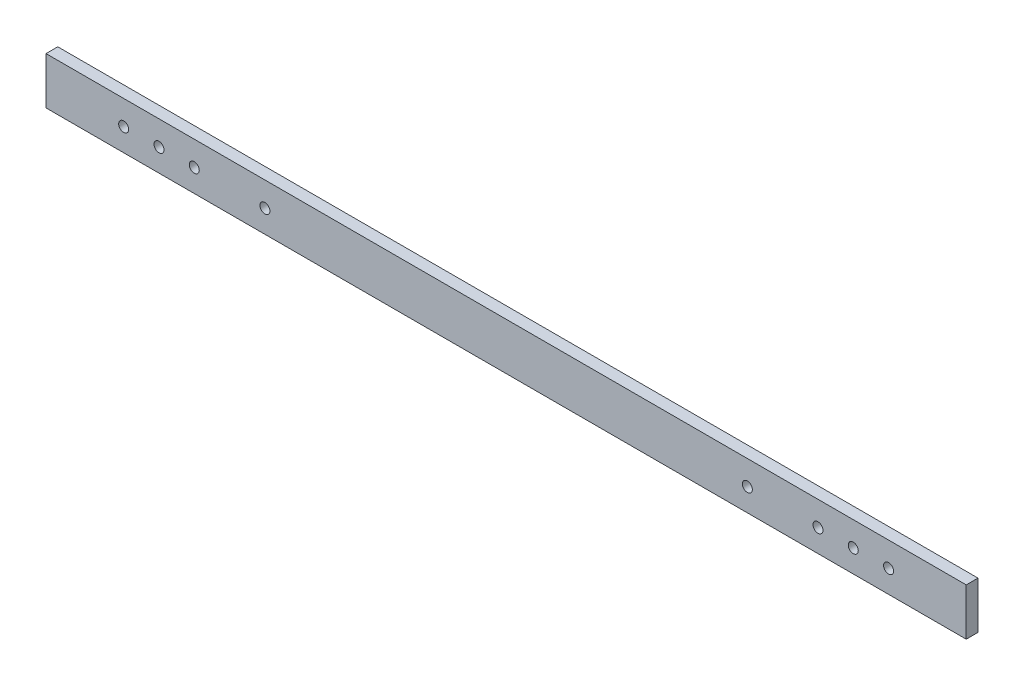
SolidWorks part; units mm, degrees
material "1023 carbon steel plate (SS)"
ref_plane "Front Plane" through (0, 0, 0) normal (0, 0, 1) x (1, 0, 0)
ref_plane "Top Plane" through (0, 0, 0) normal (0, 1, 0) x (1, 0, 0)
ref_plane "Right Plane" through (0, 0, 0) normal (1, 0, 0) x (0, 0, -1)
sketch "Sketch1" plane through (0, 0, 0) normal (0, 0, 1) x (1, 0, 0)
  line L1 (391, 20) -> (-391, 20)
  line L2 (391, 20) -> (391, -20)
  line L3 (391, -20) -> (-391, -20)
  line L4 (-391, 20) -> (-391, -20)
  line L5 (391, 20) -> (-391, -20) construction
  line L6 (391, -20) -> (-391, 20) construction
  point P0 (0, 0)
  dimension "D1" = 782
  dimension "D2" = 40
extrude "Boss-Extrude1" add sketch "Sketch1" along normal blind 10
sketch "Sketch2" plane through (0, 0, 10) normal (0, 0, 1) x (1, 0, 0)
  line L0 (-391, 20) -> (-391, -20) construction
  line L1 (0, 0) -> (0, 76.6808) construction
  line L2 (391, 20) -> (-391, 20) construction
  circle A0 centre (-325, -0.78) radius 4
  circle A1 centre (-295, -0.78) radius 4
  circle A2 centre (-265, -0.78) radius 4
  circle A3 centre (-205, -0.78) radius 4
  circle A12 centre (205, -0.78) radius 4
  circle A13 centre (265, -0.78) radius 4
  circle A14 centre (295, -0.78) radius 4
  circle A15 centre (325, -0.78) radius 4
  dimension "D1" = 8
  dimension "D6" = 20.78
  dimension "D2" = 30
  dimension "D3" = 66
  dimension "D4" = 30
  dimension "D5" = 60
hole_wizard "M10 Tapped Hole3" positions "Sketch7" profile "Sketch8" tap size "M10" standard "ISO"
sketch "Sketch7" plane through (0, 0, 10) normal (0, 0, 1) x (1, 0, 0)
  point P0 (-325, -0.78)
  point P3 (-295, -0.78)
  point P6 (-265, -0.78)
  point P9 (-205, -0.78)
  point P12 (205, -0.78)
  point P15 (265, -0.78)
  point P18 (295, -0.78)
  point P21 (325, -0.78)
sketch "Sketch8" plane through (-325, -0.78, 10) normal (1, 0, 0) x (0, -1, 0)
  line L0 (0, 0) -> (0, 27.0537)
  line L1 (0, 27.0537) -> (4.25, 24.5)
  line L2 (4.25, 24.5) -> (4.25, 0)
  line L5 (4.25, 0) -> (0, 0)
  line L10 (0, 27.0537) -> (-4.25, 24.5) construction
  line L11 (0, -6.35) -> (0, 107.95) construction
  dimension "螺纹孔钻头直径" = 8.5
  dimension "螺纹孔钻头深度" = 24.5
  dimension "导头角度" = 118
cosmetic thread "Cosmetic thread 19"
cosmetic thread "Cosmetic thread 20"
cosmetic thread "Cosmetic thread 21"
cosmetic thread "Cosmetic thread 22"
cosmetic thread "Cosmetic thread 23"
cosmetic thread "Cosmetic thread 24"
cosmetic thread "Cosmetic thread 25"
cosmetic thread "Cosmetic thread 26"
